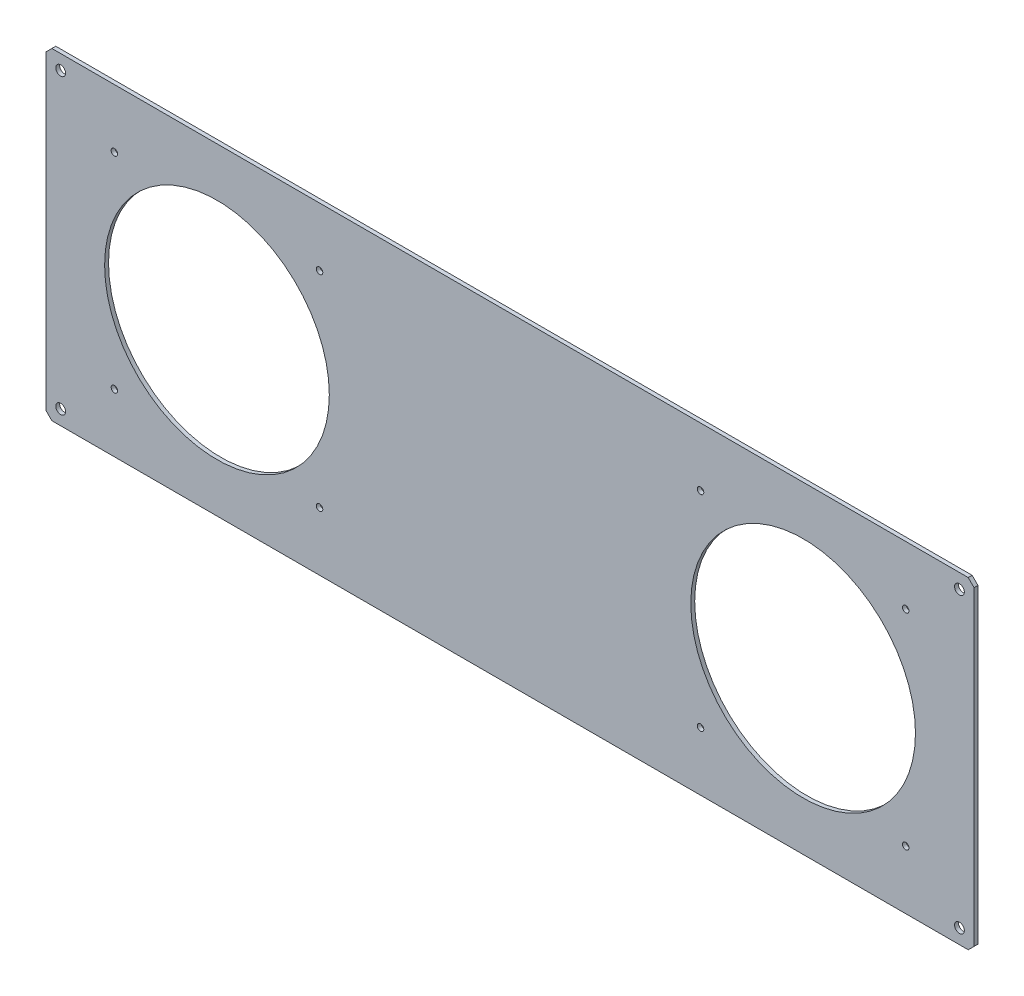
SolidWorks part; units mm, degrees
ref_plane "前视" through (0, 0, 0) normal (0, 0, 1) x (1, 0, 0)
ref_plane "上视" through (0, 0, 0) normal (0, 1, 0) x (1, 0, 0)
ref_plane "右视" through (0, 0, 0) normal (1, 0, 0) x (0, 0, -1)
sketch "草图1" plane through (0, 0, 0) normal (0, 0, 1) x (1, 0, 0)
  line L1 (-237.5, 82.5) -> (237.5, 82.5)
  line L2 (-237.5, 82.5) -> (-237.5, -82.5)
  line L3 (-237.5, -82.5) -> (237.5, -82.5)
  line L4 (237.5, 82.5) -> (237.5, -82.5)
  line L5 (-237.5, 82.5) -> (237.5, -82.5) construction
  line L6 (-237.5, -82.5) -> (237.5, 82.5) construction
  point P0 (0, 0)
  dimension "D1" = 475
  dimension "D2" = 165
extrude "凸台-拉伸1" add sketch "草图1" along normal blind 2
hole_wizard "Ø5.0 (5) 直径孔1" positions "草图3" profile "草图2" hole size "Ø5.0" standard "Iso" end condition through all
sketch "草图3" plane through (0, 0, 2) normal (0, 0, 1) x (1, 0, 0)
  line L0 (0, 0) -> (0, 63.5597) construction
  line L2 (0, 0) -> (76.6978, 0) construction
  point P0 (-230, 75)
  point P2 (-230, -75)
  point P4 (230, 75)
  point P6 (230, -75)
  dimension "D1" = 460
  dimension "D2" = 150
sketch "草图2" plane through (-230, 75, 2) normal (1, 0, 0) x (0, -1, 0)
  line L0 (0, 0) -> (0, 2)
  line L1 (0, 2) -> (2.5, 2)
  line L2 (2.5, 2) -> (2.5, 0)
  line L5 (2.5, 0) -> (0, 0)
  line L11 (0, -6.35) -> (0, 107.95) construction
  dimension "通孔孔直径" = 5
  dimension "通孔孔深度" = 2
chamfer "倒角1" distance 3 angle 45 4 edges at (237.5, 82.5, 1) (237.5, -82.5, 1) (-237.5, -82.5, 1) (-237.5, 82.5, 1)
sketch "草图4" plane through (0, 0, 2) normal (0, 0, 1) x (1, 0, 0)
  line L0 (0, 0) -> (0, 67.2662) construction
  line L1 (0, 0) -> (106.2402, 0) construction
  circle A0 centre (-150, 0) radius 57.5
  circle A1 centre (150, 0) radius 57.5
  dimension "D1" = 115
  dimension "D2" = 300
extrude "切除-拉伸1" cut sketch "草图4" against normal blind 2
hole_wizard "M4 螺纹孔1" positions "草图6" profile "草图5" tap size "M4" standard "Iso"
sketch "草图6" plane through (0, 0, 2) normal (0, 0, 1) x (1, 0, 0)
  line L0 (-150, 0) -> (150, 0) construction
  line L2 (-150, 0) -> (-150, 121.5411) construction
  line L4 (150, 0) -> (150, 100.1776) construction
  point P0 (-202.5, 52.5)
  point P2 (-97.5, 52.5)
  point P4 (-97.5, -52.5)
  point P6 (-202.5, -52.5)
  point P8 (97.5, -52.5)
  point P10 (202.5, -52.5)
  point P12 (202.5, 52.5)
  point P14 (97.5, 52.5)
  dimension "D1" = 105
  dimension "D2" = 105
  dimension "D3" = 105
sketch "草图5" plane through (-202.5, 52.5, 2) normal (1, 0, 0) x (0, -1, 0)
  line L0 (0, 0) -> (0, 11.0914)
  line L1 (0, 11.0914) -> (1.65, 10.1)
  line L2 (1.65, 10.1) -> (1.65, 0)
  line L5 (1.65, 0) -> (0, 0)
  line L10 (0, 11.0914) -> (-1.65, 10.1) construction
  line L11 (0, -6.35) -> (0, 107.95) construction
  dimension "螺纹孔钻头直径" = 3.3
  dimension "螺纹孔钻头深度" = 10.1
  dimension "导头角度" = 118
